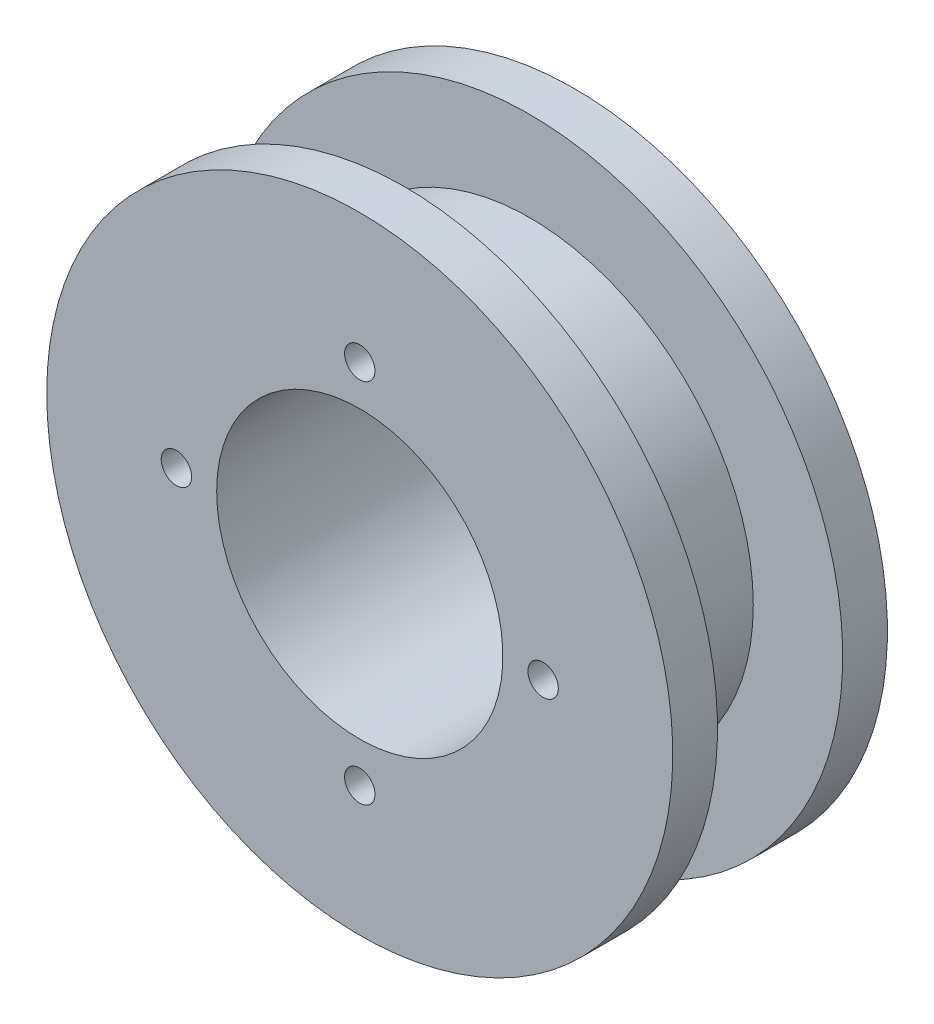
from build123d import *

# Parameters (mm, degrees)
HOLE_WIZARD_M8_1_D     = 6.8
HOLE_WIZARD_M8_1_DEPTH = 19.75
HOLE_WIZARD_M8_1_TIP   = 2.042926105
HOLE_WIZARD_M8_3_D     = 6.8
HOLE_WIZARD_M8_3_DEPTH = 19.75
HOLE_WIZARD_M8_3_TIP   = 2.042926105


with BuildPart() as part:
    # 草图1 → 旋转1 (revolve)
    with BuildSketch(Plane(origin=(0, 0, 0), x_dir=(1, 0, 0), z_dir=(0, 1, 0))):
        Polygon((-32, 48), (-70, 48), (-70, 38), (-50, 38), (-50, 10), (-70, 10), (-70, 0), (-32, 0), align=None)
    revolve(axis=Axis((0, 0, 0), (0, 0, 1)))

    # M8 螺纹孔1
    with Locations(Plane(origin=(0, 0, -48), x_dir=(-1, 0, 0), z_dir=(0, 0, -1))):
        with Locations((0, 41), (41, 0), (-41, 0), (0, -41)):
            Hole(HOLE_WIZARD_M8_1_D / 2, depth=HOLE_WIZARD_M8_1_DEPTH)
            with Locations((0, 0, -(HOLE_WIZARD_M8_1_DEPTH + HOLE_WIZARD_M8_1_TIP / 2))):  # 118° drill point
                Cone(0, HOLE_WIZARD_M8_1_D / 2, HOLE_WIZARD_M8_1_TIP, mode=Mode.SUBTRACT)

    # M8 螺纹孔3
    with Locations(Plane.XY):
        with Locations((41, 0), (0, -41), (-41, 0), (0, 41)):
            Hole(HOLE_WIZARD_M8_3_D / 2, depth=HOLE_WIZARD_M8_3_DEPTH)
            with Locations((0, 0, -(HOLE_WIZARD_M8_3_DEPTH + HOLE_WIZARD_M8_3_TIP / 2))):  # 118° drill point
                Cone(0, HOLE_WIZARD_M8_3_D / 2, HOLE_WIZARD_M8_3_TIP, mode=Mode.SUBTRACT)


solid = part.part
